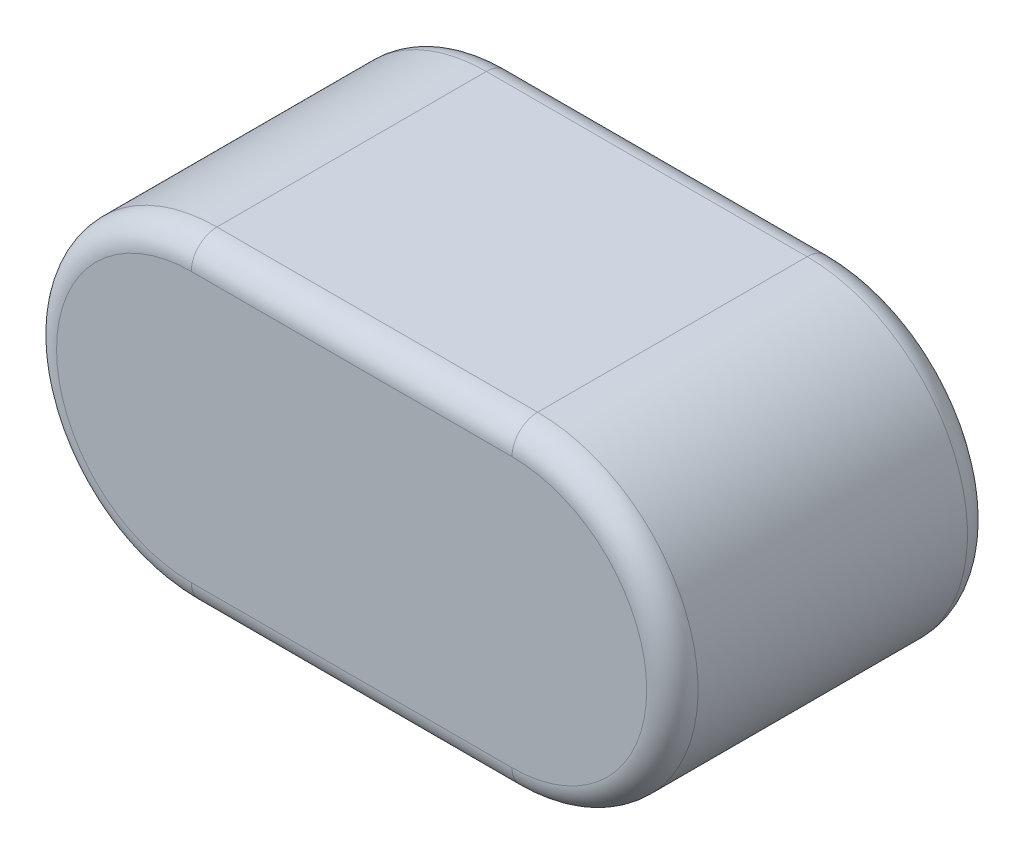
from build123d import *

# Parameters (mm, degrees)
EXTRUDE_527_DEPTH = 5
FILLET_1_R        = 0.4


with BuildPart() as part:
    # 草图1 → Extrude 527 (new body)
    with BuildSketch(Plane.XY):
        with BuildLine():
            Line((-2.5, 2.5), (2.5, 2.5))
            ThreePointArc((2.5, 2.5), (5, 0), (2.5, -2.5))
            Line((2.5, -2.5), (-2.5, -2.5))
            ThreePointArc((-2.5, -2.5), (-5, 0), (-2.5, 2.5))
        make_face()
    extrude(amount=EXTRUDE_527_DEPTH)

    # 圆角1
    fillet_1_edges = [part.edges().sort_by_distance(p)[0] for p in [
        (5, 0, 5),
        (0, 2.5, 5),
        (-5, 0, 5),
        (0, 2.5, 0),
        (5, 0, 0),
        (0, -2.5, 0),
        (-5, 0, 0),
        (0, -2.5, 5),
    ]]
    fillet(fillet_1_edges, radius=FILLET_1_R)


solid = part.part
